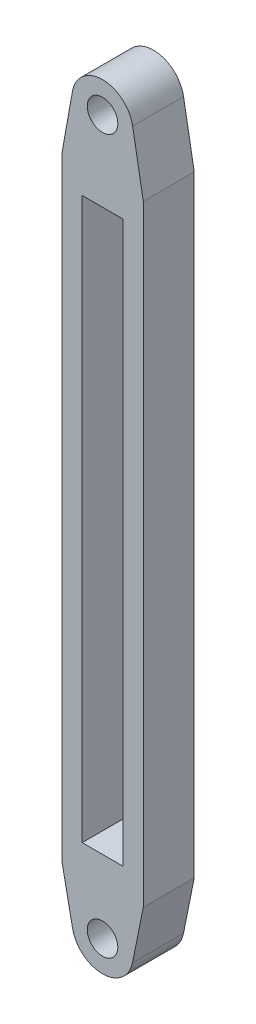
from build123d import *

# Parameters (mm, degrees)
SKETCH1_R           = 3
SKETCH1_W           = 8
SKETCH1_H           = 110
BOSS_EXTRUDE1_DEPTH = 10


with BuildPart() as part:
    # Sketch1 → Boss-Extrude1 (new body)
    with BuildSketch(Plane.XY):
        with BuildLine():
            Line((2.118738771, -10.491083349), (0, 0))
            Line((0, 0), (0, 120))
            Line((0, 120), (2.092997217, 131.74896535))
            ThreePointArc((2.092997217, 131.74896535), (8, 136.696673509), (13.907002783, 131.74896535))
            Line((13.907002783, 131.74896535), (16, 120))
            Line((16, 120), (16, 0))
            Line((16, 0), (13.881261229, -10.491083349))
            ThreePointArc((13.881261229, -10.491083349), (8, -15.303326491), (2.118738771, -10.491083349))
        make_face()
        with Locations((8, 130.696673509)):
            Circle(SKETCH1_R, mode=Mode.SUBTRACT)
        with Locations((8, -9.303326491)):
            Circle(SKETCH1_R, mode=Mode.SUBTRACT)
        with Locations((8, 60)):
            Rectangle(SKETCH1_W, SKETCH1_H, mode=Mode.SUBTRACT)
    extrude(amount=BOSS_EXTRUDE1_DEPTH)


solid = part.part
